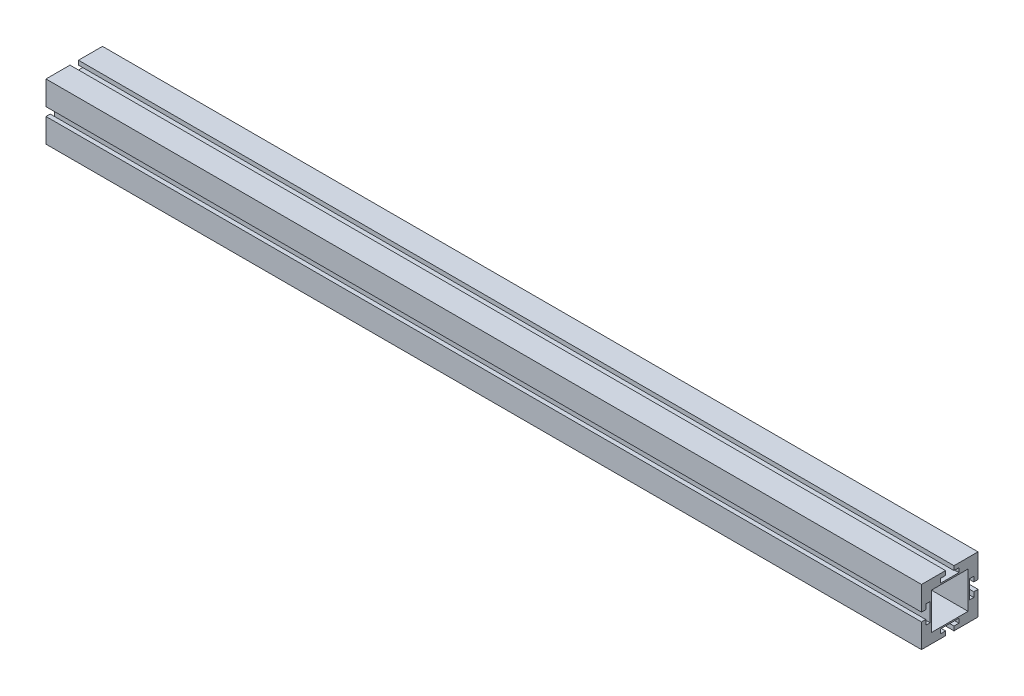
from build123d import *

# Parameters (mm, degrees)
SKETCH1_W           = 26
SKETCH1_H           = 26
BOSS_EXTRUDE1_DEPTH = 620


with BuildPart() as part:
    # Sketch1 → Boss-Extrude1 (new body)
    with BuildSketch(Plane(origin=(0, 0, 0), x_dir=(0, 0, -1), z_dir=(1, 0, 0))):
        Polygon((-20, -20), (-3, -20), (-3, -17), (-6.5, -17), (-6.5, -14), (6.5, -14), (6.5, -17), (3, -17), (3, -20), (20, -20), (20, -3), (17, -3), (17, -6.5), (14, -6.5), (14, 6.5), (17, 6.5), (17, 3), (20, 3), (20, 20), (3, 20), (3, 17), (6.5, 17), (6.5, 14), (-6.5, 14), (-6.5, 17), (-3, 17), (-3, 20), (-20, 20), (-20, 3), (-17, 3), (-17, 6.5), (-14, 6.5), (-14, -6.5), (-17, -6.5), (-17, -3), (-20, -3), align=None)
        Rectangle(SKETCH1_W, SKETCH1_H, mode=Mode.SUBTRACT)
    extrude(amount=BOSS_EXTRUDE1_DEPTH)


solid = part.part
